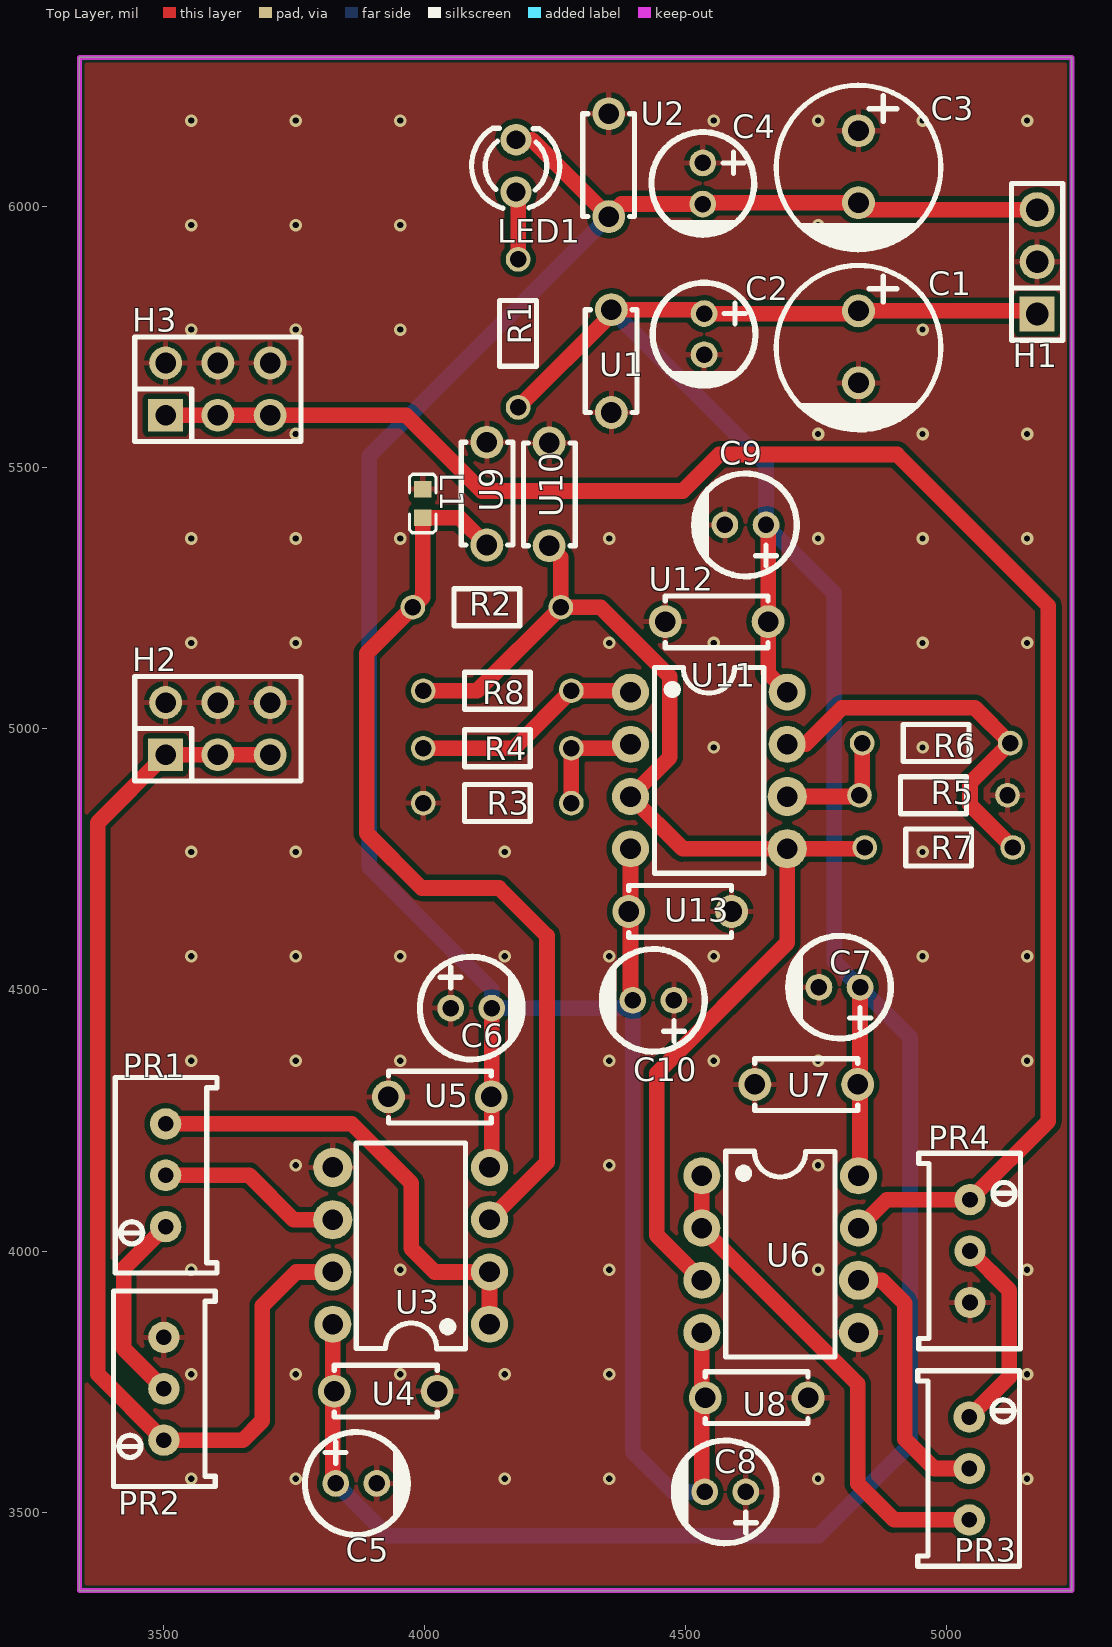
[diagram p0: Top Layer view]
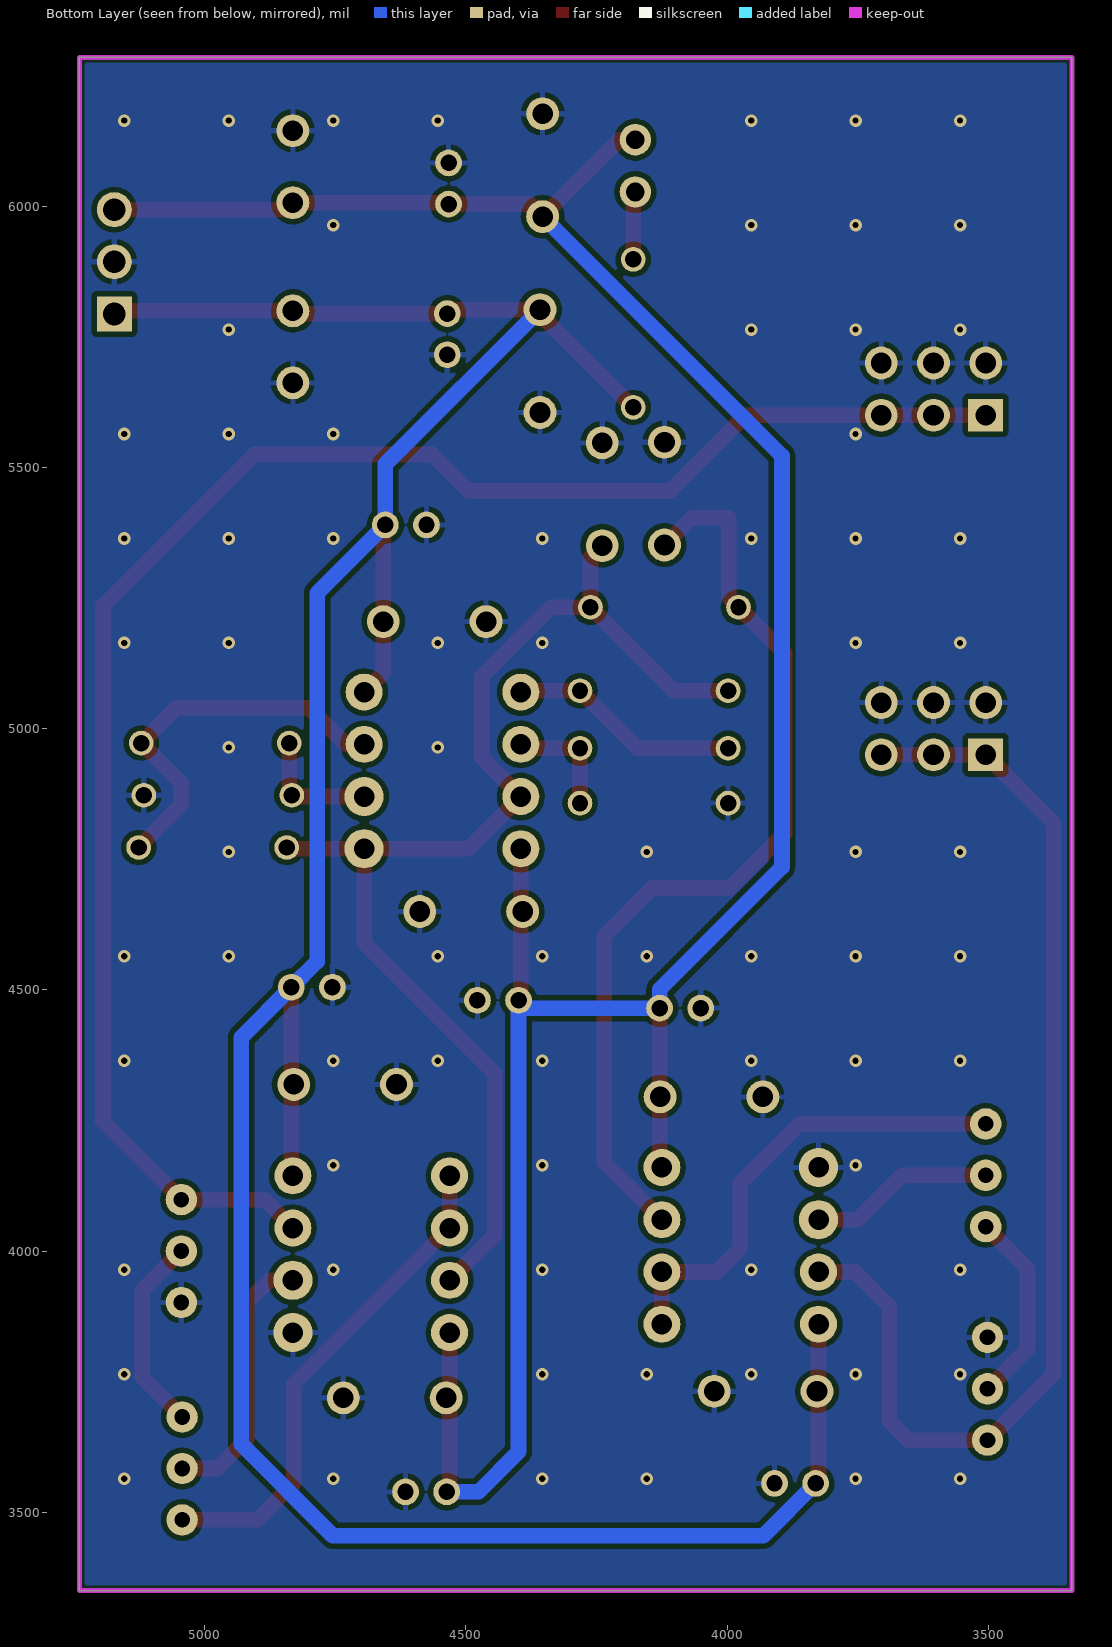
[diagram p1: Bottom Layer view, seen from below]
# Altium PCB MISC51743.pcbdoc
Units mil, origin at the board's own origin, x right, y up, seen from the top; angles counter-clockwise.
Board outline 1900 x 2935 mil, 2 copper layers (Top Layer, Bottom Layer), stack 62.206 mil thick; 40 components, 18 nets, 111 pads, 73 vias.

## Layer stack, top to bottom
Top Solder Mask Layer: solder mask 0.394, Dk 3.3
Top Layer: signal copper 1.379
Dielectric1: surface 59.449, FR4, Dk 4.5
Bottom Layer: signal copper 1.378
Bottom Solder Mask Layer: solder mask 0.394, Dk 3.3

## Board outline
3340,6285 3340,3350 5240,3350 5240,6285

## Design rules (kind name [scope] priority, off if disabled: settings)
BoardOutlineClearance copperThickness2oz_1 [All] p2 off: genericclearance=7.99 ignorepadtopadclearanceinfootprint=FALSE except(0: Arc-SplitContinuation Track-SplitContinuation SMDPad-SplitContinuation THPad-SplitContinuation Via-SplitContinuation Fill-SplitContinuation Region-SplitContinuation Poly-SplitContinuation Text-SplitContinuation Hole-SplitContinuation; 5.98: Arc-CutoutEdge SMDPad-CutoutEdge THPad-CutoutEdge Via-CutoutEdge Fill-CutoutEdge Region-CutoutEdge Text-CutoutEdge; 6.93: Hole-OutlineEdge Hole-CutoutEdge; 10: Poly-OutlineEdge Poly-CutoutEdge; 11.81: Arc-OutlineEdge Track-OutlineEdge SMDPad-OutlineEdge THPad-OutlineEdge Via-OutlineEdge Fill-OutlineEdge Region-OutlineEdge Text-OutlineEdge Track-CutoutEdge)
BoardOutlineClearance copperThickness1oz_1 [All] p4: genericclearance=4.02 ignorepadtopadclearanceinfootprint=FALSE except(0: Arc-SplitContinuation Track-SplitContinuation SMDPad-SplitContinuation THPad-SplitContinuation Via-SplitContinuation Fill-SplitContinuation Region-SplitContinuation Poly-SplitContinuation Text-SplitContinuation Hole-SplitContinuation; 6: SMDPad-CutoutEdge THPad-CutoutEdge Via-CutoutEdge Fill-CutoutEdge Region-CutoutEdge Text-CutoutEdge; 6.93: Hole-OutlineEdge Hole-CutoutEdge; 10: Poly-OutlineEdge Poly-CutoutEdge; 11.8: Arc-OutlineEdge Track-OutlineEdge SMDPad-OutlineEdge THPad-OutlineEdge Via-OutlineEdge Fill-OutlineEdge Region-OutlineEdge Text-OutlineEdge; 11.81: Arc-CutoutEdge Track-CutoutEdge)
Clearance copperThickness2oz [All] p1 off: gap=7.99 ignorepadtopadclearanceinfootprint=FALSE except(5.98: SMDPad-Track SMDPad-SMDPad THPad-Track SMDPad-THPad THPad-THPad Track-Via SMDPad-Via THPad-Via Via-Via Fill-Track Region-Track Fill-SMDPad Region-SMDPad Fill-THPad Region-THPad Fill-Via Region-Via Fill-Fill Fill-Region Region-Region Arc-Track Arc-SMDPad Arc-THPad Arc-Via Fill-Arc Region-Arc Arc-Arc Text-Track SMDPad-Text Text-THPad Text-Via Fill-Text Region-Text Arc-Text Text-Text; 6.93: Hole-Track Hole-SMDPad Hole-THPad Hole-Via Fill-Hole Region-Hole Hole-Arc Hole-Text; 10: Poly-Track Poly-SMDPad Poly-THPad Poly-Via Poly-Fill Poly-Region Poly-Poly Poly-Arc Poly-Text Poly-Hole)
Clearance copperThickness1oz [All] p3: gap=4.02 ignorepadtopadclearanceinfootprint=FALSE except(5.98: SMDPad-Track SMDPad-SMDPad THPad-Track SMDPad-THPad THPad-THPad Track-Via SMDPad-Via THPad-Via Via-Via Fill-Track Region-Track Fill-SMDPad Region-SMDPad Fill-THPad Region-THPad Fill-Via Region-Via Fill-Fill Fill-Region Region-Region; 6: Arc-Track Arc-SMDPad Arc-THPad Arc-Via Fill-Arc Region-Arc Arc-Arc Text-Track SMDPad-Text Text-THPad Text-Via Fill-Text Region-Text Arc-Text Text-Text; 6.93: Hole-Track Hole-SMDPad Hole-THPad Hole-Via Fill-Hole Region-Hole Hole-Arc Hole-Text; 10: Poly-Track Poly-SMDPad Poly-THPad Poly-Via Poly-Fill Poly-Region Poly-Poly Poly-Arc Poly-Text Poly-Hole)
Creepage creepage [All] p1: checkdistance=0 ignoreinternallayers=TRUE applytopolygonpour=TRUE
DiffPairsRouting differentialPair [All] p1: maxlimit=6 minlimit=6 mostfreqgap=6 toplayer_minwidth=5 toplayer_prefwidth=10 toplayer_maxwidth=100 toplayer_mingap=6 toplayer_prefgap=6 toplayer_maxgap=6 bottomlayer_minwidth=5 bottomlayer_prefwidth=10 bottomlayer_maxwidth=100 bottomlayer_mingap=6 bottomlayer_prefgap=6 bottomlayer_maxgap=6 maxuncoupledlength=10
HoleToHoleClearance otherClearance [All] p1: gap=11.81 allowstackedmicrovias=TRUE
Length netLength [All] p1: minlimit=0 maxlimit=0
MatchedLengths netLengthTolerance [All] p1: tolerance=1000
PasteMaskExpansion pasteMaskExpansion [All] p1: expansion=0
PlaneConnect innerPlane [All] p1: planeconnectstyle=Relief reliefexpansion=20 reliefentries=4 reliefconductorwidth=10 reliefairgap=10
PolygonConnect copperRegion [(InNet('GND'))] p1: connectstyle=Relief reliefconductorwidth=10 reliefentries=4 polygonreliefangle="90 Angle" airgapwidth=10 via.connectstyle=Relief via.reliefconductorwidth=10 via.reliefentries=4 via.polygonreliefangle="90 Angle" via.airgapwidth=10
RoutingVias viaSize [All] p1: holewidth=12.01 width=24.02 viastyle="Through Hole" minholewidth=11.81 minwidth=19.68 maxholewidth=248.03 maxwidth=393.7
SolderMaskExpansion solderMaskExpansion [IsVia] p1: expansion=-1000 istentingtop=TRUE
SolderMaskExpansion solderMaskExpansion [All] p2: expansion=2 istentingtop=FALSE
Width copperThickness2oz_2 [All] p1 off: maxlimit=100 minlimit=8 preferedwidth=10
Width copperThickness1oz_2 [All] p2: maxlimit=100 minlimit=5 preferedwidth=10

## Components (designator, comment, footprint, x,y, rotation, side; value= is the part's Value field where it differs from the comment)
C1 "100uF" CAP-TH_BD8.0-P3.50-D0.6-FD_1 4831.41,5730.89 r270 top
C2 "10uF" CAP-TH_BD5.0-P2.00-D0.8-FD-10UF50VC110GL 4535.79,5755.26 r270 top
C3 "100uF" CAP-TH_BD8.0-P3.50-D0.6-FD_1 4831.41,6075.84 r270 top
C4 "10uF" CAP-TH_BD5.0-P2.00-D0.8-FD-10UF50VC110GL 4533.33,6043.74 r270 top
C5 "10uF" CAP-TH_BD5.0-P2.00-D0.8-FD-10UF50VC110GL 3870,3555 r0 top
C6 "10uF" CAP-TH_BD5.0-P2.00-D0.8-FD-10UF50VC110GL 4090,4465 r0 top
C7 "10uF" CAP-TH_BD5.0-P2.00-D0.8-FD-10UF50VC110GL 4795,4505 r180 top
C8 "10uF" CAP-TH_BD5.0-P2.00-D0.8-FD-10UF50VC110GL 4576.4,3538.91 r180 top
C9 "10uF" CAP-TH_BD5.0-P2.00-D0.8-FD-10UF50VC110GL 4615,5390 r180 top
C10 "10uF" CAP-TH_BD5.0-P2.00-D0.8-FD-10UF50VC110GL 4438.74,4480 r180 top
H1 "" HDR-TH_3P-P2.54-V-M 5173.33,5893.74 r90 top
H2 "" HDR-TH_6P-P2.54-V-F-R2-C3-S2.54 3605,5000 r0 top
H3 "" HDR-TH_6P-P2.54-V-F-R2-C3-S2.54 3605,5650 r0 top
L1 "20mH" L0603 3997.22,5431.11 r270 top
LED1 "" LED_TH-3mm 4175.79,6077.46 r90 top
PR1 "5kΩ" R_3296 3500,4145 r90 top
PR2 "200Ω" R_3296 3496.6,3736.3 r90 top
PR3 "5kΩ" R_3296 5048.4,3583.7 r270 top
PR4 "200Ω" R_3296 5050,4000 r270 top
R1 "20kΩ" Res_1/8W 4182.26,5756.63 r90 top
R2 "10kΩ" Res_1/8W 4120,5230 r0 top
R3 "10kΩ" Res_1/8W 4140,4855 r0 top
R4 "10kΩ" Res_1/8W 4140,4965 r180 top
R5 "10kΩ" Res_1/8W 4975,4875 r180 top
R6 "10kΩ" Res_1/8W 4980,4970 r0 top
R7 "10kΩ" Res_1/8W 4985,4775 r180 top
R8 "10kΩ" Res_1/8W 4140,5075 r180 top
U1 "100nF" CAP-TH_L5.0-W2.5-P5.00-D1.0 4358.33,5703.74 r270 top
U2 "100nF" CAP-TH_L5.0-W2.5-P5.00-D1.0 4353.33,6078.74 r270 top
U3 "NE5532AP" PDIP-8_L9.6-W6.4-P2.54-LS7.6-BL 3975,4010 r90 top
U4 "100nF" CAP-TH_L5.0-W2.5-P5.00-D1.0 3926.4,3731.39 r180 top
U5 "100nF" CAP-TH_L5.0-W2.5-P5.00-D1.0 4030,4295 r0 top
U6 "NE5532AP" PDIP-8_L9.6-W6.4-P2.54-LS7.6-BL 4681.4,3993.91 r270 top
U7 "100nF" CAP-TH_L5.0-W2.5-P5.00-D1.0 4731.4,4318.91 r0 top
U8 "100nF" CAP-TH_L5.0-W2.5-P5.00-D1.0 4636.4,3718.91 r180 top
U9 "100nF" CAP-TH_L5.0-W2.5-P5.00-D1.0 4120,5450 r90 top
U10 "100nF" CAP-TH_L5.0-W2.5-P5.00-D1.0 4239.19,5448.67 r90 top
U11 "NE5532AP" PDIP-8_L9.6-W6.4-P2.54-LS7.6-BL 4545,4920 r270 top
U12 "100nF" CAP-TH_L5.0-W2.5-P5.00-D1.0 4560,5205 r0 top
U13 "100nF" CAP-TH_L5.0-W2.5-P5.00-D1.0 4490,4650 r180 top

## Footprints (in the part's own frame and the unit in brackets; to place one, negate y for a bottom-side part, rotate by r counter-clockwise, add the part's x,y. Pads: shape width x height; smd on the part's side, far side on the other; paste and mask are expansions set on the pad)
CAP-TH_BD5.0-P2.00-D0.8-FD-10UF50VC110GL [mm]
  round 1.3 hole 0.8: 1(-1,0) 2(1,0)
  silkscreen extent -2.5,-2.5 2.5,2.5
CAP-TH_BD8.0-P3.50-D0.6-FD_1 [mm]
  round 1.6 hole 1: 1(-1.75,0) 2(1.75,0)
  silkscreen extent -3.96,-4 4.04,4
CAP-TH_L5.0-W2.5-P5.00-D1.0 [mm]
  round 1.6 hole 1: 1(-2.5,0) 2(2.5,0)
  silkscreen extent -2.5,-1.27 2.5,1.25
HDR-TH_3P-P2.54-V-M [mm]
  rect 1.7x1.7 hole 1.1: 1(-2.54,0)
  round 1.7 hole 1.1: 2(0,0) 3(2.54,0)
  silkscreen extent -3.81,-1.25 3.81,1.25
HDR-TH_6P-P2.54-V-F-R2-C3-S2.54 [mm]
  rect 1.7x1.6 hole 1: 1(-2.54,-1.27)
  round 1.6 hole 1: 2(-2.54,1.27) 3(0,-1.27) 4(0,1.27) 5(2.54,-1.27) 6(2.54,1.27)
  silkscreen extent -4.04,-2.54 4.04,2.54
L0603 [mm]
  rect 0.8x0.864 smd paste-100 mask+0.051: 1(-0.7,0) 2(0.7,0)
  silkscreen extent -1.42,-0.65 1.42,0.65
LED_TH-3mm [mil]
  round 60 hole 36 paste+0 mask+2: 1(-50,0) 2(50,0)
  silkscreen extent -81,-84 72,85
PDIP-8_L9.6-W6.4-P2.54-LS7.6-BL [mm]
  round 1.8 hole 1: 1(-3.81,-3.81) 2(-1.27,-3.81) 3(1.27,-3.81) 4(3.81,-3.81) 7(-1.27,3.81) 8(-3.81,3.81)
  round 1.905 hole 1: 5(3.81,3.81) 6(1.27,3.81)
  silkscreen extent -5,-2.64 5,2.67
R_3296 [mil]
  round 60 hole 30 paste+0 mask+2: 1(-98.4,-5) 2(0,-5) 3(98.4,-5)
  silkscreen extent -187,-103 187,92
Res_1/8W [mil]
  round 47.2 hole 31.5 paste+0 mask+2: 1(-141.7,2.48) 2(141.7,2.48)
  silkscreen extent -63,-33 63,38

## Via types
v1: diameter 24.02, hole 12, Top Layer to Bottom Layer, 73 vias

## Nets (pads, with @x,y where several pads share a name; then routed paths per layer and width w, separated by ;. In a path a pad name is that pad's centre, name@x,y a point inside that pad or via, vN(x,y) a via of type N, cw(c..) or ccw(c..) an arc to the next point about the centre after c; other vN are vias at no path point)
$1N5: LED1.1 R1.2 | length 130.8
  Top Layer w30: LED1.1 4179.78,6023.47 R1.2
$1N19: PR1.2 U3.6 | length 355.2
  Top Layer w30: PR1.2 3665,4145 3750,4060 U3.6
$1N21: PR1.1 PR2.2 | length 375.2
  Top Layer w30: PR2.2 3425,3812.9 3425,3966.6 PR1.1
$1N26: PR3.1 PR4.2 | length 380.7
  Top Layer w30: PR3.1 5120,3758.7 5120,3925 PR4.2
$1N28: PR3.2 U6.6 | length 513.5
  Top Layer w30: U6.6 4876.09,3943.91 4920,3900 4920,3640 4976.3,3583.7 PR3.2
$1N44: R3.2 R4.1 U11.2 | length 221.4
  Top Layer w30: R3.2 R4.1 4387.52,4962.52 U11.2
$1N45: R4.2 R8.1 U11.1 | length 443.3
  Top Layer w30: R4.2 4171.7,4962.52 R8.1 4392.48,5072.52 U11.1
$1N47: R5.2 R6.1 U11.6 | length 241.4
  Top Layer w30: U11.6 4830.78,4870 R5.2 4838.3,4877.52 R6.1
$1N48: R6.2 R7.1 U11.7 | length 749.2
  Top Layer w30: U11.7 4730,4970 4800,5040 5054.18,5040 R6.2 5045,4895.78 5045,4854.22 R7.1
+12V: C1.1 C2.1 C5.1 C7.1 C9.1 H1.1 R1.1 U1.1 U3.8 U4.2 U6.8 U7.2 U11.8 U12.2 | length 5712.7
  Top Layer w30: U3.8 3825,3560.63 C5.1 ; R1.1 4358.33,5793.48 U1.1 4528.26,5802.16 C2.1 4826.25,5794.63 C1.1 5167.27,5799.79 H1.1 ; C9.1 4658.43,5385.94 U12.2 4658.43,5106.57 U11.8 ; U6.8 4834.37,4146.88 C7.1
  Bottom Layer w30: C5.1 3930.63,3455 4755,3455 4930,3630 4930,4409.37 C7.1 4785,4554.37 4785,5259.37 C9.1 4654.37,5506.12 U1.1
-12V: C3.2 C4.2 C6.2 C8.2 C10.2 H1.3 LED1.2 U2.2 U3.4 U5.2 U6.4 U8.2 U11.4 U13.2 | length 5093.2
  Top Layer w30: U3.4 4129.37,4164.37 C6.2 ; LED1.2 4206.18,6127.46 U2.2 4377.38,6004.37 C4.2 4535.9,6006.94 C3.2 4844.61,5993.74 H1.3 ; U11.4 4395,4484.37 C10.2 ; U6.4 4531.4,3544.54 C8.2
  Bottom Layer w30: U2.2 3895,5521.99 3895,4735 4129.37,4500.63 C6.2 4384.37,4465 C10.2 4399.37,3615.63 4476.09,3538.91 C8.2
GND: C1.2 C2.2 C3.1 C4.1 C5.2 C6.1 C7.2 C8.1 C9.2 C10.1 H1.2 H2.2 H2.4 H2.6 H3.2 H3.4 H3.6 L1.1 PR2.3 PR4.3 R3.1 R5.1 U1.2 U2.1 U3.5 U4.1 U5.1 U6.5 U7.1 U8.1 U9.2 U10.2 U12.1 U13.1
  other v1: 3554.1,3564.1 3754.1,3564.1 4154.1,3564.1 4354.1,3564.1 4754.1,3564.1 5154.1,3564.1 3554.1,3764.1 3754.1,3764.1 3954.1,3764.1 4154.1,3764.1 4354.1,3764.1 5154.1,3764.1 3554.1,3964.1 3954.1,3964.1 4354.1,3964.1 4754.1,3964.1 5154.1,3964.1 3754.1,4164.1 4354.1,4164.1 4754.1,4164.1 3554.1,4364.1 3754.1,4364.1 3954.1,4364.1 4354.1,4364.1 4554.1,4364.1 4754.1,4364.1 5154.1,4364.1 3554.1,4564.1 3754.1,4564.1 3954.1,4564.1 4154.1,4564.1 4354.1,4564.1 4554.1,4564.1 4954.1,4564.1 5154.1,4564.1 3554.1,4764.1 3754.1,4764.1 4154.1,4764.1 4954.1,4764.1 4554.1,4964.1 4954.1,4964.1 3554.1,5164.1 3754.1,5164.1 4354.1,5164.1 4554.1,5164.1 4954.1,5164.1 5154.1,5164.1 3554.1,5364.1 3754.1,5364.1 3954.1,5364.1 4354.1,5364.1 4754.1,5364.1 4954.1,5364.1 5154.1,5364.1 3754.1,5564.1 4754.1,5564.1 4954.1,5564.1 5154.1,5564.1 3554.1,5764.1 3754.1,5764.1 3954.1,5764.1 4954.1,5764.1 3554.1,5964.1 3754.1,5964.1 3954.1,5964.1 4754.1,5964.1 3554.1,6164.1 3754.1,6164.1 3954.1,6164.1 4554.1,6164.1 4754.1,6164.1 4954.1,6164.1 5154.1,6164.1
X1: L1.2 R2.1 U3.3 U9.1 | length 1807.6
  Top Layer w30: U9.1 4068.02,5403.56 L1.2 3997.22,5251.4 R2.1 3890,5144.18 3890,4800 3995,4695 4143.25,4695 4235,4603.25 4235,4170 U3.3
X2: PR1.3 U3.1 U3.2 | length 910.6
  Top Layer w30: PR1.3 3861.6,4243.4 3975,4130 3975,4005 4020,3960 U3.2 U3.1
X3: H2.1 H2.3 H2.5 PR2.1 U3.7 | length 2204.1
  Top Layer w30: H2.5 H2.3 H2.1 3375,4820 3375,3764.5 PR2.1 3652.9,3637.9 3690,3675 3690,3895 3755,3960 U3.7
Y1: R2.2 R7.2 R8.2 U6.3 U10.1 U11.3 U11.5 | length 2437.2
  Top Layer w30: R8.2 4101.75,5072.52 R2.2 ; U10.1 4261.7,5327.73 R2.2 ; U6.3 4445,4030.3 4445,4340 4695,4590 U11.5 ; R7.2 4840.78,4770 U11.5 ; R2.2 4337.52,5232.48 4470,5100 4470,4945 U11.3 4495,4770 U11.5
Y2: PR3.3 U6.1 U6.2 | length 954.9
  Top Layer w30: U6.1 U6.2 4830,3745.3 4830,3555 4899.7,3485.3 PR3.3
Y3: H3.1 H3.3 H3.5 PR4.1 U6.7 | length 3334.1
  Top Layer w30: H3.1 H3.3 H3.5 3965,5600 4110,5455 4495,5455 4565,5525 4905,5525 5195,5235 5195,4248.4 PR4.1 4885.89,4098.4 U6.7

## Polygon pours and split planes (outlines as drawn)
GND on Top Layer (solid, remove dead copper, pour order 0): 3055,6535 3055,3000 5575,3000 5575,6535
GND on Bottom Layer (solid, remove dead copper, pour order 2): 3000,6445 3000,3125 5675,3125 5675,6445

## Keep-outs
Board Outline Layer:
  the board outline again, w10